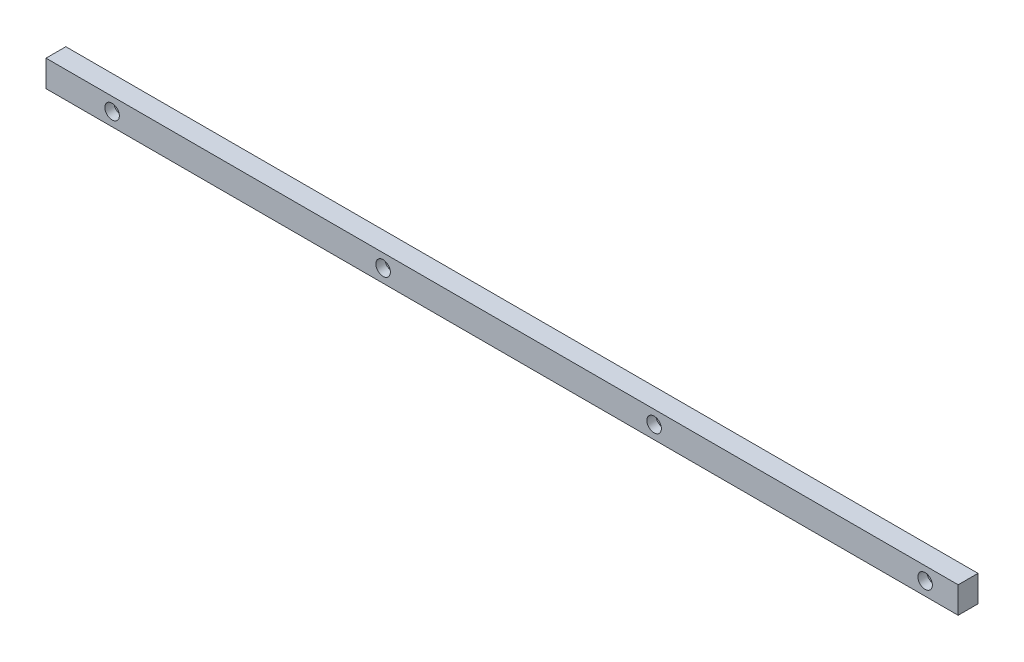
SolidWorks part; units mm, degrees
ref_plane "前视基准面" through (0, 0, 0) normal (0, 0, 1) x (1, 0, 0)
ref_plane "上视基准面" through (0, 0, 0) normal (0, 1, 0) x (1, 0, 0)
ref_plane "右视基准面" through (0, 0, 0) normal (1, 0, 0) x (0, 0, -1)
sketch "草图1" plane through (0, 0, 0) normal (0, 0, 1) x (1, 0, 0)
  line L1 (-332.5, 10) -> (332.5, 10)
  line L2 (-332.5, 10) -> (-332.5, -10)
  line L3 (-332.5, -10) -> (332.5, -10)
  line L4 (332.5, 10) -> (332.5, -10)
  line L5 (-332.5, 10) -> (332.5, -10) construction
  line L6 (-332.5, -10) -> (332.5, 10) construction
  point P0 (0, 0)
  dimension "D1" = 20
  dimension "D2" = 665
extrude "凸台-拉伸1" add sketch "草图1" along normal blind 15
hole_wizard "打孔尺寸(%根据)内六角圆柱头螺钉的类型1" positions "草图2" profile "草图4" counterbore size "M6" standard "GB" end condition through all
sketch "草图2" plane through (0, 0, 15) normal (0, 0, 1) x (1, 0, 0)
  line L0 (-307.5, 0) -> (0, 0) construction
  line L1 (0, 0) -> (307.5, 0) construction
  line L3 (0, 0) -> (0, 67.8719) construction
  point P11 (-307.5, 0)
  point P14 (307.5, 0)
  point P21 (-102.5, 0)
  point P29 (102.5, 0)
  dimension "D1" = 205
  dimension "D2" = 205
sketch "草图4" plane through (102.5, 0, 15) normal (1, 0, 0) x (0, -1, 0)
  line L0 (0, 0) -> (0, 15)
  line L1 (0, 15) -> (3.3, 15)
  line L3 (3.3, 15) -> (3.3, 6.8)
  line L4 (3.3, 6.8) -> (5.5, 6.8)
  line L5 (5.5, 6.8) -> (5.5, 0)
  line L7 (5.5, 0) -> (0, 0)
  line L11 (0, -6.35) -> (0, 107.95) construction
  dimension "通孔孔直径" = 6.6
  dimension "通孔孔深度" = 15
  dimension "柱形沉头孔直径" = 11
  dimension "柱形沉头孔深度" = 6.8
sketch "草图5" plane through (-332.5, 0, 0) normal (-1, 0, 0) x (0, 0, 1)
  line L4 (0, 10) -> (0, -10)
  line L5 (0, -10) -> (15, -10)
  line L6 (15, -10) -> (15, 10)
  line L7 (15, 10) -> (0, 10)
  line L8 (0, 10) -> (0, -10)
  line L9 (0, -10) -> (15, -10)
  line L10 (15, -10) -> (15, 10)
  line L11 (15, 10) -> (0, 10)
  dimension "D1" = 0
extrude "凸台-拉伸2" add sketch "草图5" along normal blind 25
